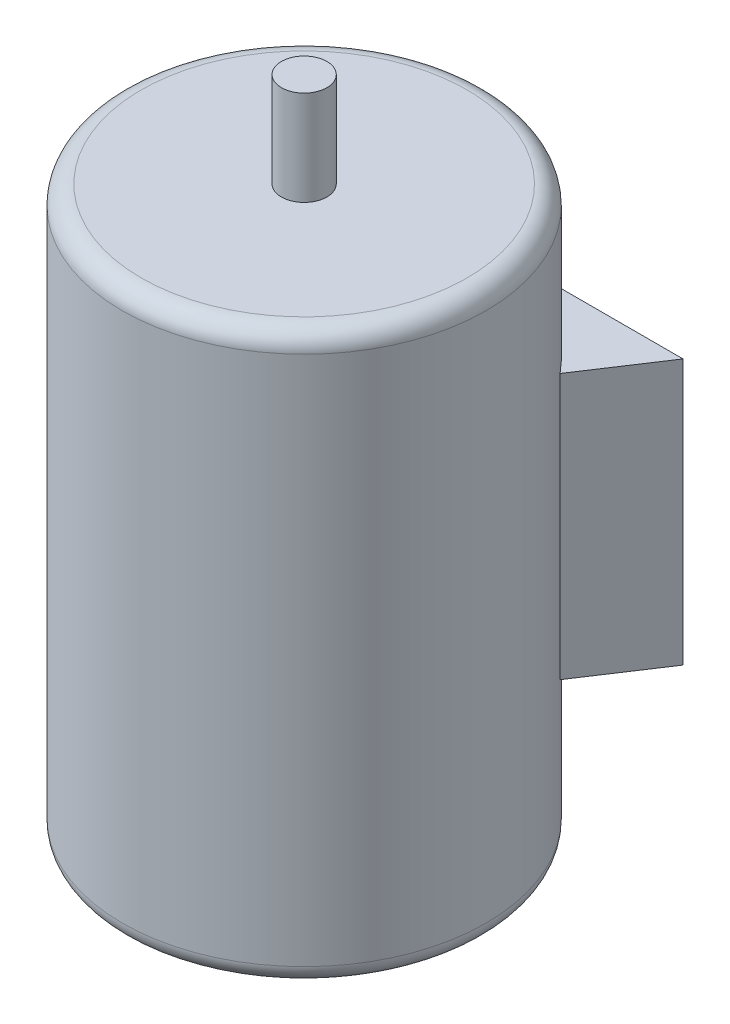
SolidWorks part; units mm, degrees
ref_plane "Front" through (0, 0, 0) normal (0, 0, 1) x (1, 0, 0)
ref_plane "Top" through (0, 0, 0) normal (0, 1, 0) x (1, 0, 0)
ref_plane "Right" through (0, 0, 0) normal (1, 0, 0) x (0, 0, -1)
sketch "Sketch1" plane through (0, 0, 0) normal (0, 1, 0) x (1, 0, 0)
  circle A0 centre (0, 0) radius 96
  dimension "D1" = 192
extrude "Boss-Extrude1" add sketch "Sketch1" along normal blind 300
sketch "Sketch2" plane through (0, 300, 0) normal (0, 1, 0) x (1, 0, 0)
  circle A0 centre (0, 0) radius 12
  dimension "D1" = 24
extrude "Boss-Extrude2" add sketch "Sketch2" along normal blind 50
fillet "Fillet1" radius 10 2 edges at (0, 0, 96) (0, 300, 96)
ref_plane "Plane1" through (0, 80, 0) normal (0, -1, 0) x (-1, 0, 0)
sketch "Sketch3" plane through (0, 80, 0) normal (0, -1, 0) x (-1, 0, 0)
  line L0 (74.2255, 60.8817) -> (100, 100)
  line L1 (100, 100) -> (-100, 100)
  line L2 (-100, 100) -> (-74.2255, 60.8817)
  circle A0 centre (0, 0) radius 96 construction
  arc A1 (74.2255, 60.8817) -> (-74.2255, 60.8817) centre (0, 0) ccw
  point P4 (0, 100)
  dimension "D1" = 200
  dimension "D2" = 0
  dimension "D3" = 100
extrude "Boss-Extrude3" add sketch "Sketch3" against normal blind 140
